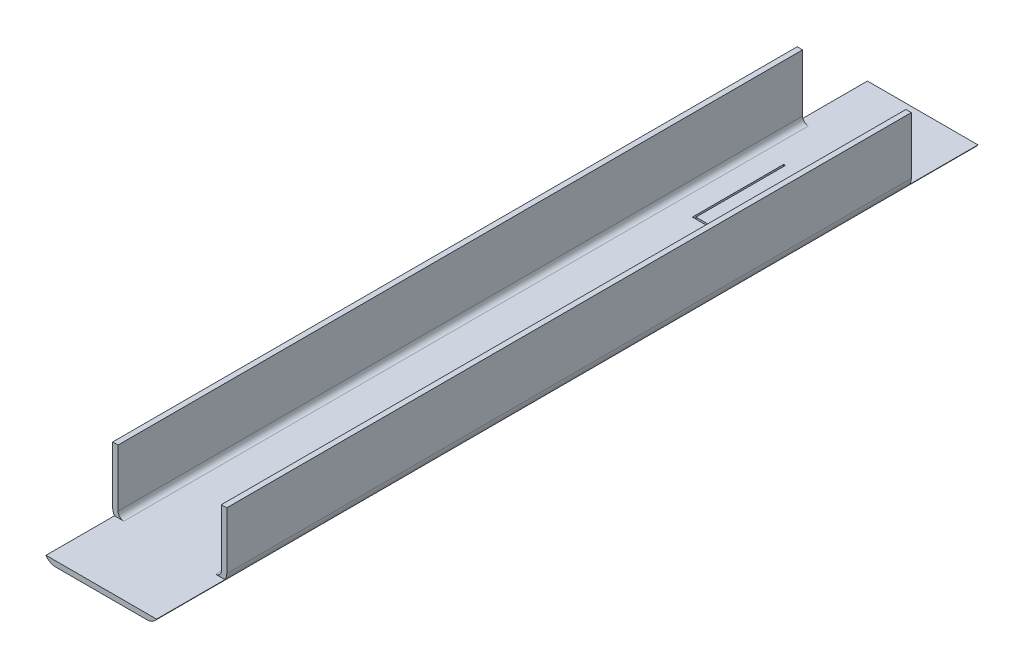
SolidWorks part; units mm, degrees
ref_plane "Front Plane" through (0, 0, 0) normal (0, 0, 1) x (1, 0, 0)
ref_plane "Top Plane" through (0, 0, 0) normal (0, 1, 0) x (1, 0, 0)
ref_plane "Right Plane" through (0, 0, 0) normal (1, 0, 0) x (0, 0, -1)
sketch "Sketch1" plane through (0, 0, 0) normal (0, 0, 1) x (1, 0, 0)
  line L0 (30.25, 3.1) -> (30.25, 19.05)
  line L1 (3.2, 0) -> (28.55, 0)
  line L2 (0, 3.2) -> (0, 19.05)
  line L3 (3.1, 1.5) -> (28.65, 1.5)
  line L4 (31.75, 3.2) -> (31.75, 19.05)
  line L5 (1.5, 3.1) -> (1.5, 19.05)
  line L6 (1.5, 19.05) -> (0, 19.05)
  line L7 (31.75, 19.05) -> (30.25, 19.05)
  line L8 (1.5, 1.5) -> (30.25, 1.5) construction
  line L9 (1.5, 1.5) -> (1.5, 19.05) construction
  line L10 (30.25, 1.5) -> (30.25, 19.05) construction
  line L11 (31.75, 0) -> (31.75, 19.05) construction
  line L12 (0, 0) -> (31.75, 0) construction
  line L13 (0, 0) -> (0, 19.05) construction
  arc A0 (3.1, 1.5) -> (1.5, 3.1) centre (3.1, 3.1) cw
  arc A1 (28.65, 1.5) -> (30.25, 3.1) centre (28.65, 3.1) ccw
  arc A2 (31.75, 3.2) -> (28.55, 0) centre (28.55, 3.2) cw
  arc A3 (0, 3.2) -> (3.2, 0) centre (3.2, 3.2) ccw
  dimension "D4" = 1.6
  dimension "D5" = 1.6
  dimension "D6" = 3.2
  dimension "D7" = 3.2
  dimension "D2" = 31.75
  dimension "D3" = 1.5
extrude "Boss-Extrude1" add sketch "Sketch1" along normal blind 228.6
sketch "Sketch2" plane through (0, 0, 0) normal (1, 0, 0) x (0, 0, -1)
  line L0 (0, 3.2) -> (0, 19.05) construction
  line L1 (0, 1.5) -> (0, 19.05)
  line L2 (-228.6, 3.2) -> (-228.6, 19.05) construction
  line L3 (-228.6, 1.5) -> (-228.6, 19.05)
  line L4 (-228.6, 1.5) -> (0, 1.5) construction
  line L5 (-228.6, 1.5) -> (-209.55, 1.5)
  line L6 (-209.55, 1.5) -> (-209.55, 19.05)
  line L7 (-228.6, 3.2) -> (-228.6, 19.05) construction
  line L8 (-209.55, 3.2) -> (-209.55, 19.05) construction
  line L9 (-19.05, 1.5) -> (-19.05, 19.05)
  line L10 (0, 3.2) -> (0, 19.05) construction
  line L11 (-19.05, 3.2) -> (-19.05, 19.05) construction
  line L12 (-19.05, 1.5) -> (0, 1.5)
  line L13 (-19.05, 19.05) -> (0, 19.05)
  line L14 (-228.6, 19.05) -> (-209.55, 19.05)
  dimension "D1" = 19.05
  dimension "D2" = 19.05
extrude "Cut-Extrude1" cut sketch "Sketch2" along normal through all
sketch "Sketch3" plane through (0, 0, 0) normal (0, 1, 0) x (1, 0, 0)
  line L1 (22.8218, -57.15) -> (8.9282, -57.15)
  line L2 (9.4282, -31.75) -> (9.4282, -56.65)
  line L3 (22.3218, -56.65) -> (9.4282, -56.65)
  line L4 (15.875, 0) -> (15.875, -77.307) construction
  line L5 (31.2611, 0) -> (0.4889, 0) construction
  line L6 (8.9282, -31.75) -> (8.9282, -57.15)
  line L7 (22.8218, -31.75) -> (22.8218, -57.15)
  line L8 (22.3218, -31.75) -> (22.3218, -56.65)
  line L9 (9.4282, -31.75) -> (8.9282, -31.75)
  line L10 (22.8218, -31.75) -> (22.3218, -31.75)
  point P0 (31.2611, -57.15)
  point P1 (0.4889, -57.15)
  point P2 (31.2611, -31.75)
  point P3 (0.4889, -31.75)
  dimension "D1" = 0.5
extrude "Cut-Extrude2" cut sketch "Sketch3" along normal through all
